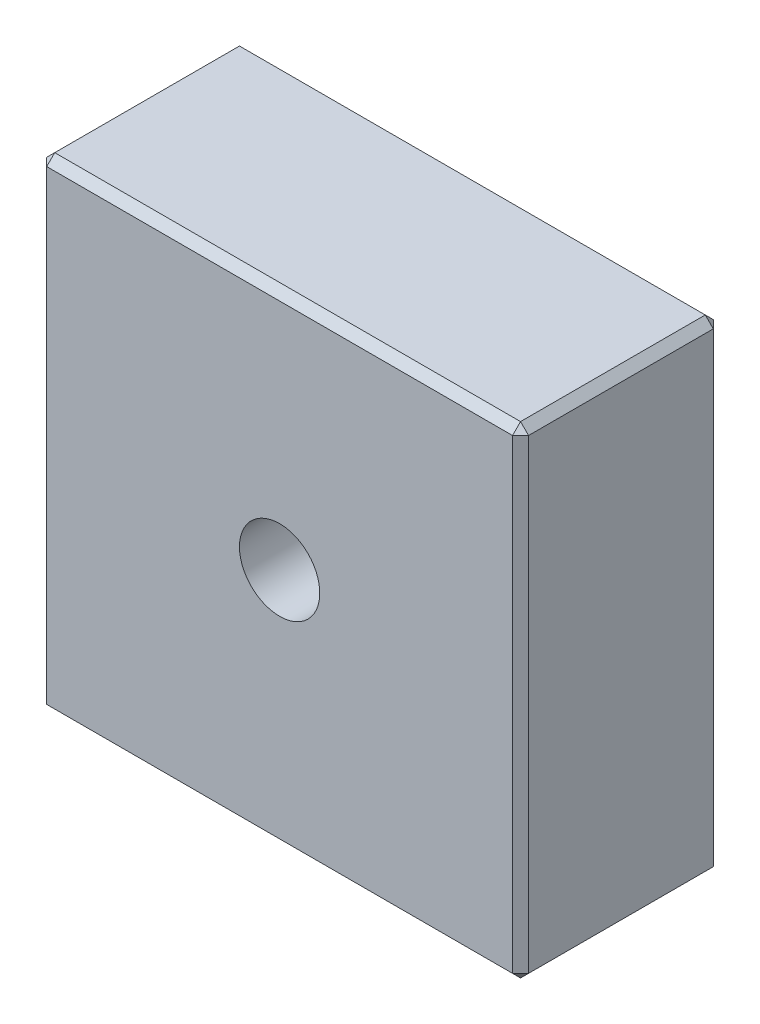
SolidWorks part; units mm, degrees
ref_plane "Front Plane" through (0, 0, 0) normal (0, 0, 1) x (1, 0, 0)
ref_plane "Top Plane" through (0, 0, 0) normal (0, 1, 0) x (1, 0, 0)
ref_plane "Right Plane" through (0, 0, 0) normal (1, 0, 0) x (0, 0, -1)
sketch "Sketch1" plane through (0, 0, 0) normal (0, 0, 1) x (1, 0, 0)
  line L1 (-30, -30) -> (30, -30)
  line L2 (-30, -30) -> (-30, 30)
  line L3 (-30, 30) -> (30, 30)
  line L4 (30, -30) -> (30, 30)
  line L5 (-30, -30) -> (30, 30) construction
  line L6 (-30, 30) -> (30, -30) construction
  point P0 (0, 0)
  dimension "D1" = 60
  dimension "D2" = 60
extrude "Boss-Extrude1" add sketch "Sketch1" along normal blind 25 contours L3 L4 L1 L2
chamfer "Chamfer1" distance 1 angle 45 12 edges at (30, 0, 0) (30, -30, 12.5) (0, -30, 0) (-30, -30, 12.5) (-30, 0, 0) (0, -30, 25) (-30, 0, 25) (30, 0, 25) (30, 30, 12.5) (0, 30, 0) (-30, 30, 12.5) (0, 30, 25)
sketch "Sketch2" plane through (0, 0, 0) normal (0, 0, -1) x (-1, 0, 0)
  circle A0 centre (0, 0) radius 15
  dimension "D1" = 30
extrude "Cut-Extrude1" cut sketch "Sketch2" against normal blind 7
sketch "Sketch3" plane through (0, 0, 7) normal (0, 0, -1) x (-1, 0, 0)
  circle A0 centre (0, 0) radius 5
  dimension "D1" = 10
extrude "Cut-Extrude2" cut sketch "Sketch3" against normal through all
